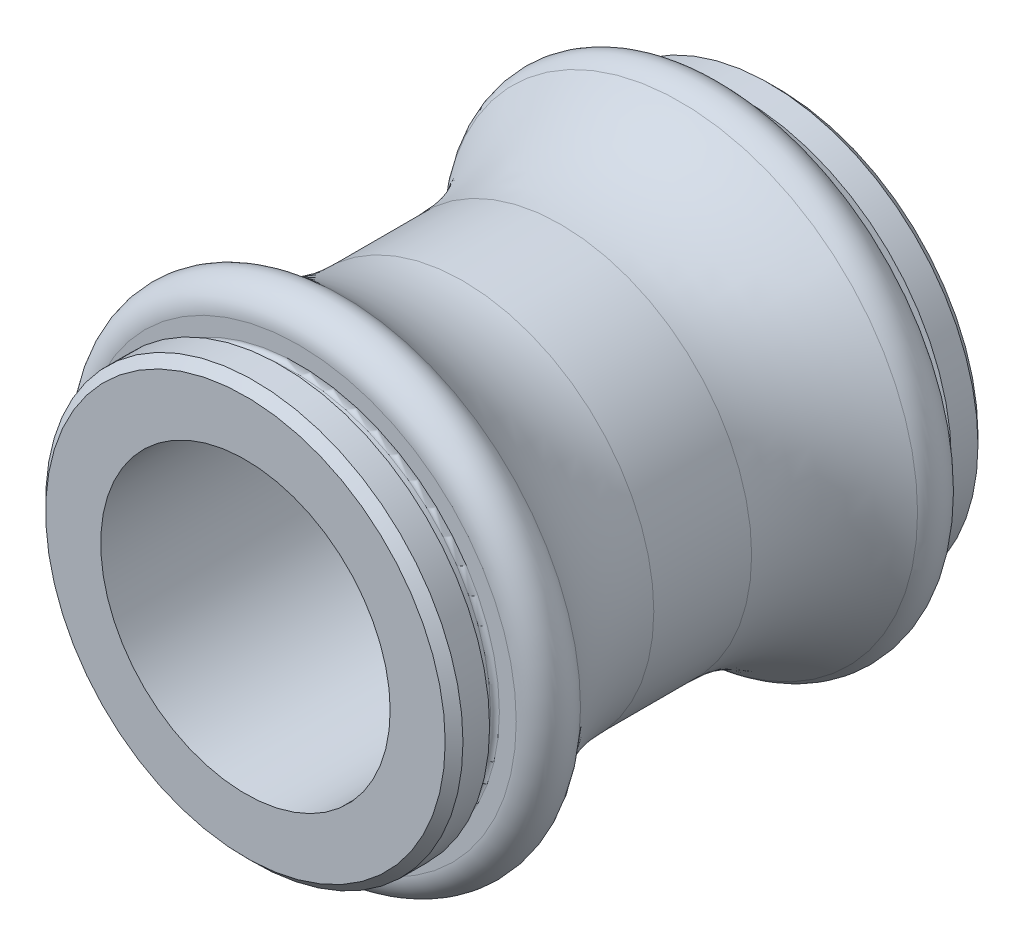
from build123d import *


with BuildPart() as part:
    # 草图1 → 旋转1 (revolve)
    with BuildSketch(Plane(origin=(0, 0, 0), x_dir=(0, 0, -1), z_dir=(1, 0, 0)), mode=Mode.PRIVATE) as revolve_1_sk:
        with BuildLine():
            Line((-30, 11.25), (-30, 8.15))
            Line((-30, 8.15), (0, 8.15))
            Line((0, 8.15), (0, 11.25))
            Line((0, 11.25), (-0.5, 11.75))
            Line((-0.5, 11.75), (-2, 11.75))
            Line((-2, 11.75), (-2, 11.3))
            ThreePointArc((-2, 11.3), (-2.073223305, 11.123223305), (-2.25, 11.05))
            Line((-2.25, 11.05), (-2.75, 11.05))
            ThreePointArc((-2.75, 11.05), (-2.926776695, 11.123223305), (-3, 11.3))
            Line((-3, 11.3), (-3, 12.25))
            ThreePointArc((-3, 12.25), (-3.893994729, 13.622136149), (-5.510343482, 13.358695652))
            ThreePointArc((-5.510343482, 13.358695652), (-8.6343911, 11.424951918), (-12.245966692, 10.75))
            Line((-12.245966692, 10.75), (-17.754033308, 10.75))
            ThreePointArc((-17.754033308, 10.75), (-21.3656089, 11.424951918), (-24.489656518, 13.358695652))
            ThreePointArc((-24.489656518, 13.358695652), (-26.106005271, 13.622136149), (-27, 12.25))
            Line((-27, 12.25), (-27, 11.3))
            ThreePointArc((-27, 11.3), (-27.073223305, 11.123223305), (-27.25, 11.05))
            Line((-27.25, 11.05), (-27.75, 11.05))
            ThreePointArc((-27.75, 11.05), (-27.926776695, 11.123223305), (-28, 11.3))
            Line((-28, 11.3), (-28, 11.75))
            Line((-28, 11.75), (-29.5, 11.75))
            Line((-29.5, 11.75), (-30, 11.25))
        make_face()
    revolve(revolve_1_sk.sketch.rotate(Axis((0, 0, 0), (0, 0, 1)), 270), axis=Axis((0, 0, 0), (0, 0, 1)))


solid = part.part
